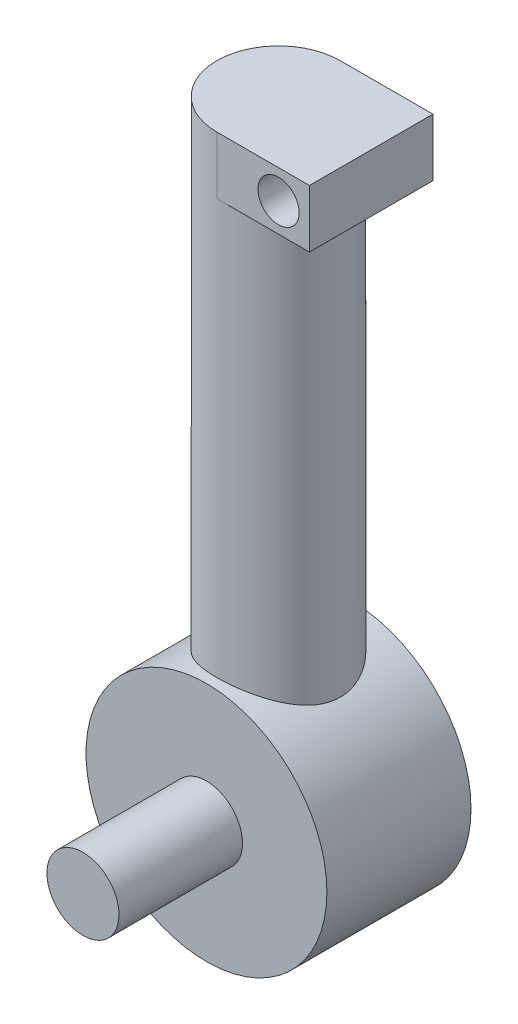
from build123d import *

# Parameters (mm, degrees)
SKETCH1_R           = 58.5
BOSS_EXTRUDE1_DEPTH = 70
SKETCH2_R           = 30
BOSS_EXTRUDE2_DEPTH = 260
BOSS_EXTRUDE4_DEPTH = 28
SKETCH7_R           = 17.5
BOSS_EXTRUDE6_DEPTH = 60
SKETCH8_R           = 10
CUT_EXTRUDE1_DEPTH  = 320.360689612


with BuildPart() as part:
    # Sketch1 → Boss-Extrude1 (new body)
    with BuildSketch(Plane.XY):
        Circle(SKETCH1_R)
    extrude(amount=BOSS_EXTRUDE1_DEPTH)

    # Sketch2 → Boss-Extrude2 (add)
    with BuildSketch(Plane(origin=(0, 0, 0), x_dir=(1, 0, 0), z_dir=(0, 1, 0))):
        with Locations(Location((0, -35, 0), (0, 0, 90))):
            Circle(SKETCH2_R)
    extrude(amount=BOSS_EXTRUDE2_DEPTH)

    # Sketch4 → Boss-Extrude4 (add)
    with BuildSketch(Plane(origin=(0, 260, 0), x_dir=(1, 0, 0), z_dir=(0, 1, 0))):
        with BuildLine():
            Line((0, -65), (45, -65))
            Line((45, -65), (45, -5))
            Line((45, -5), (0, -5))
            ThreePointArc((0, -5), (-30, -35), (0, -65))
        make_face()
    extrude(amount=BOSS_EXTRUDE4_DEPTH)

    # Sketch7 → Boss-Extrude6 (add)
    with BuildSketch(Plane.XY.offset(70)):
        Circle(SKETCH7_R)
    extrude(amount=BOSS_EXTRUDE6_DEPTH)

    # Sketch8 → Cut-Extrude1 (cut, through all)
    with BuildSketch(Plane(origin=(0, 0, 5), x_dir=(-1, 0, 0), z_dir=(0, 0, -1))):
        with Locations((-30, 274)):
            Circle(SKETCH8_R)
    extrude(amount=-CUT_EXTRUDE1_DEPTH, mode=Mode.SUBTRACT)


solid = part.part
